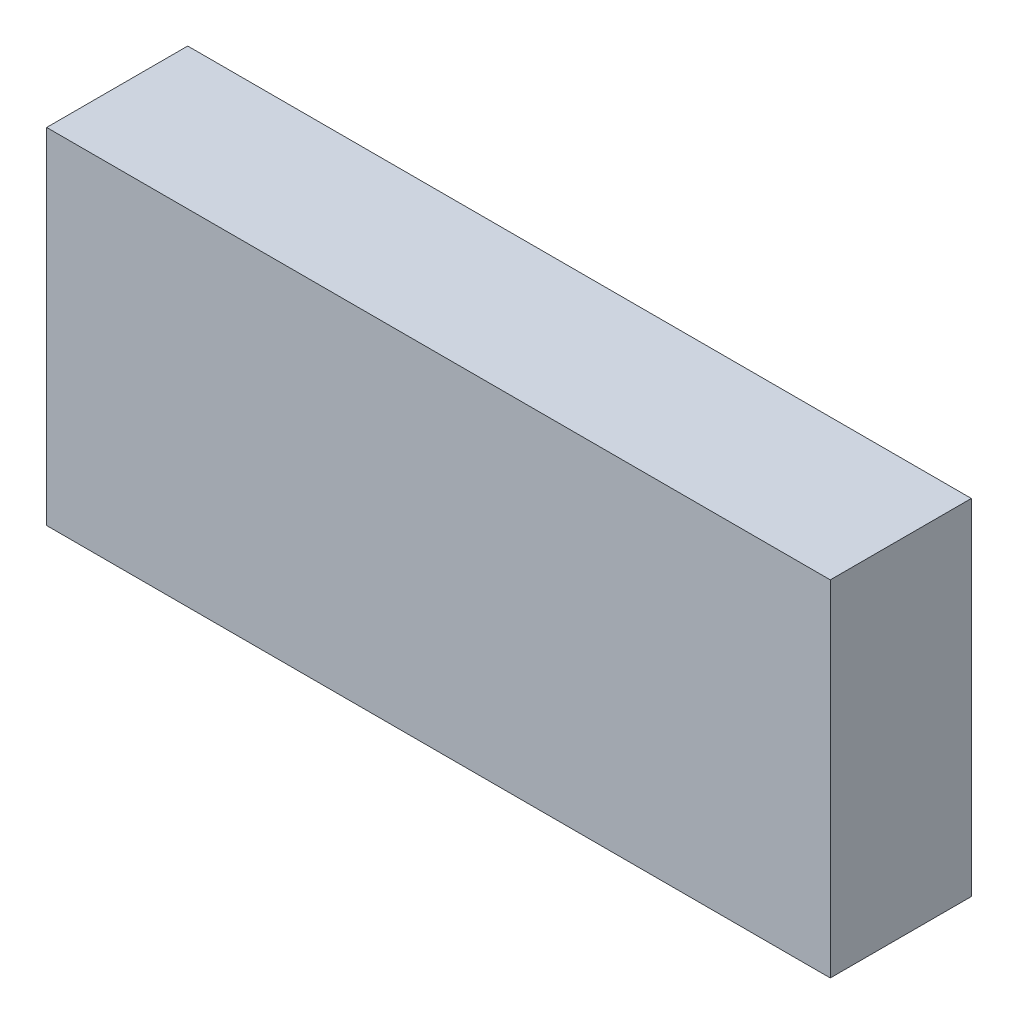
SolidWorks part; units mm, degrees
material "Q235-A"
ref_plane "Front Plane" through (0, 0, 0) normal (0, 0, 1) x (1, 0, 0)
ref_plane "Top Plane" through (0, 0, 0) normal (0, 1, 0) x (1, 0, 0)
ref_plane "Right Plane" through (0, 0, 0) normal (1, 0, 0) x (0, 0, -1)
sketch "Sketch1" plane through (0, 0, 0) normal (0, 0, 1) x (1, 0, 0)
  line L1 (125, -55) -> (-125, -55)
  line L2 (125, -55) -> (125, 55)
  line L3 (125, 55) -> (-125, 55)
  line L4 (-125, -55) -> (-125, 55)
  line L5 (125, -55) -> (-125, 55) construction
  line L6 (125, 55) -> (-125, -55) construction
  point P0 (0, 0)
  dimension "D1" = 250
  dimension "D2" = 110
extrude "Boss-Extrude1" add sketch "Sketch1" along normal mid plane 45
